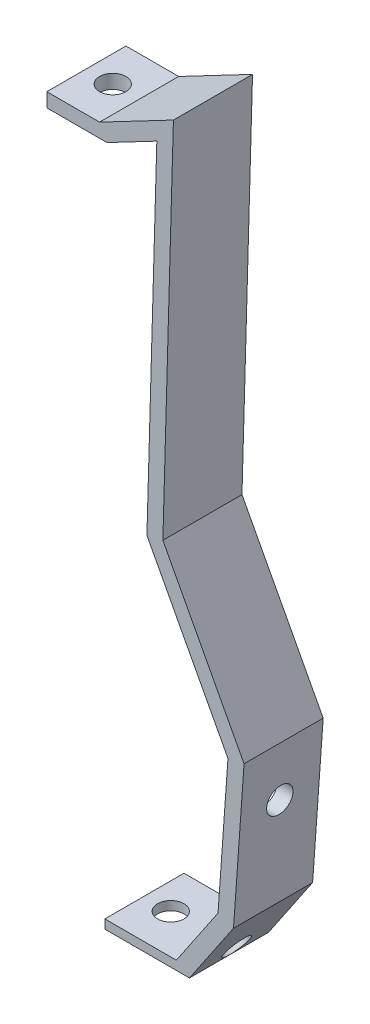
from build123d import *

# Parameters (mm, degrees)
EXTRUDE_1_DEPTH     = 7.5
SKETCH_2_W          = 11.393502177
SKETCH_2_H          = 2.656718216
SKETCH_2_W_2        = 27.04099035
SKETCH_2_H_2        = 1.681293315
EXTRUDE_2_DEPTH     = 15
SKETCH_3_R          = 2.5
CUT_EXTRUDE_1_DEPTH = 5
SKETCH_4_R          = 2.5
CUT_EXTRUDE_2_DEPTH = 10
SKETCH_5_W          = 11
SKETCH_5_H          = 15
CUT_EXTRUDE_3_DEPTH = 3
SKETCH_9_R          = 2.5


with BuildPart() as part:
    # 草图1 → 凸台-拉伸1 (new, symmetric)
    with BuildSketch(Plane.XY):
        Polygon((0, 0), (14, 7.343281784), (12, -62.656718216), (27.393502177, -91.656718216), (25.393502177, -119.656718216), (17.04099035, -132), (14.556387205, -130.318706685), (22.458397846, -118.641172307), (24.339745043, -92.302311555), (8.978589163, -63.363249125), (10.854852, 2.305950198), (1.393502177, -2.656718216), align=None)
    extrude(amount=EXTRUDE_1_DEPTH, both=True)

    # 草图2 → 凸台-拉伸2 (add)
    with BuildSketch(Plane.XY.offset(7.5)):
        with Locations((-4.303248911, -1.328359108)):
            Rectangle(SKETCH_2_W, SKETCH_2_H)
        with Locations((3.520495175, -131.159353342)):
            Rectangle(SKETCH_2_W_2, SKETCH_2_H_2)
    extrude(amount=-EXTRUDE_2_DEPTH)

    # 草图3 → 切除-拉伸1 (cut)
    with BuildSketch(Plane(origin=(0, 0, 0), x_dir=(1, 0, 0), z_dir=(0, 1, 0))):
        with Locations(Location((-5, 0, 0), (0, 0, 270))):
            Circle(SKETCH_3_R)
    extrude(amount=-CUT_EXTRUDE_1_DEPTH, mode=Mode.SUBTRACT)

    # 草图4 → 切除-拉伸2 (cut)
    with BuildSketch(Plane.XZ.offset(132)):
        with Locations(Location((6, 0, 0), (0, 0, 270))):
            Circle(SKETCH_4_R)
    extrude(amount=-CUT_EXTRUDE_2_DEPTH, mode=Mode.SUBTRACT)

    # 草图5 → 切除-拉伸3 (cut)
    with BuildSketch(Plane.XZ.offset(132)):
        with Locations((-4.5, 0)):
            Rectangle(SKETCH_5_W, SKETCH_5_H)
    extrude(amount=-CUT_EXTRUDE_3_DEPTH, mode=Mode.SUBTRACT)

    # 草图9 → 切除-旋转1 (revolve, cut)
    with BuildSketch(Plane(origin=(33.768124273, -2.412008877, 0), x_dir=(0, 0, -1), z_dir=(0.997458699830735, -0.07124704998790972, 0)), mode=Mode.PRIVATE) as cut_revolve_1_sk:
        with Locations((0, -99.543422459)):
            Circle(SKETCH_9_R)
    revolve(cut_revolve_1_sk.sketch.rotate(Axis((25.607243327, -116.664342117, 0), (0, 0, 1)), 6.860802101), axis=Axis((25.607243327, -116.664342117, 0), (0, 0, 1)), mode=Mode.SUBTRACT)


solid = part.part
